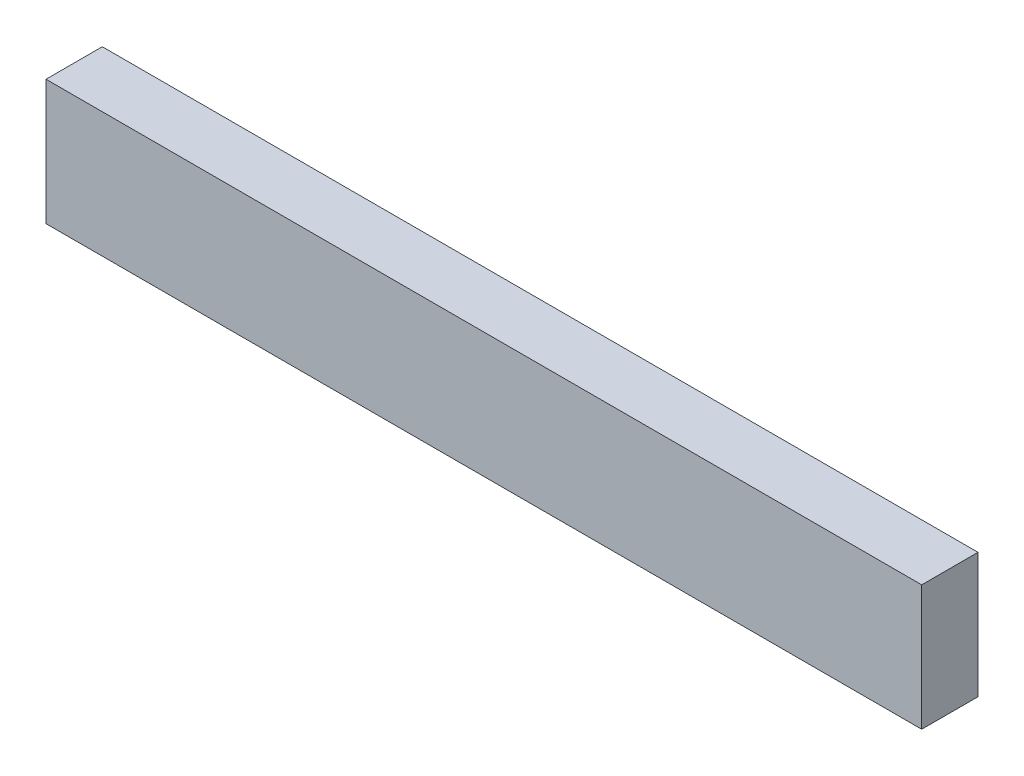
SolidWorks part; units mm, degrees
ref_plane "前视基准面" through (0, 0, 0) normal (0, 0, 1) x (1, 0, 0)
ref_plane "上视基准面" through (0, 0, 0) normal (0, 1, 0) x (1, 0, 0)
ref_plane "右视基准面" through (0, 0, 0) normal (1, 0, 0) x (0, 0, -1)
sketch "草图1" plane through (0, 0, 0) normal (0, 0, 1) x (1, 0, 0)
  line L1 (-70, -10) -> (70, -10)
  line L2 (-70, -10) -> (-70, 10)
  line L3 (-70, 10) -> (70, 10)
  line L4 (70, -10) -> (70, 10)
  line L5 (-70, -10) -> (70, 10) construction
  line L6 (-70, 10) -> (70, -10) construction
  point P0 (0, 0)
  dimension "D1" = 140
  dimension "D2" = 20
extrude "凸台-拉伸1" add sketch "草图1" along normal blind 9
